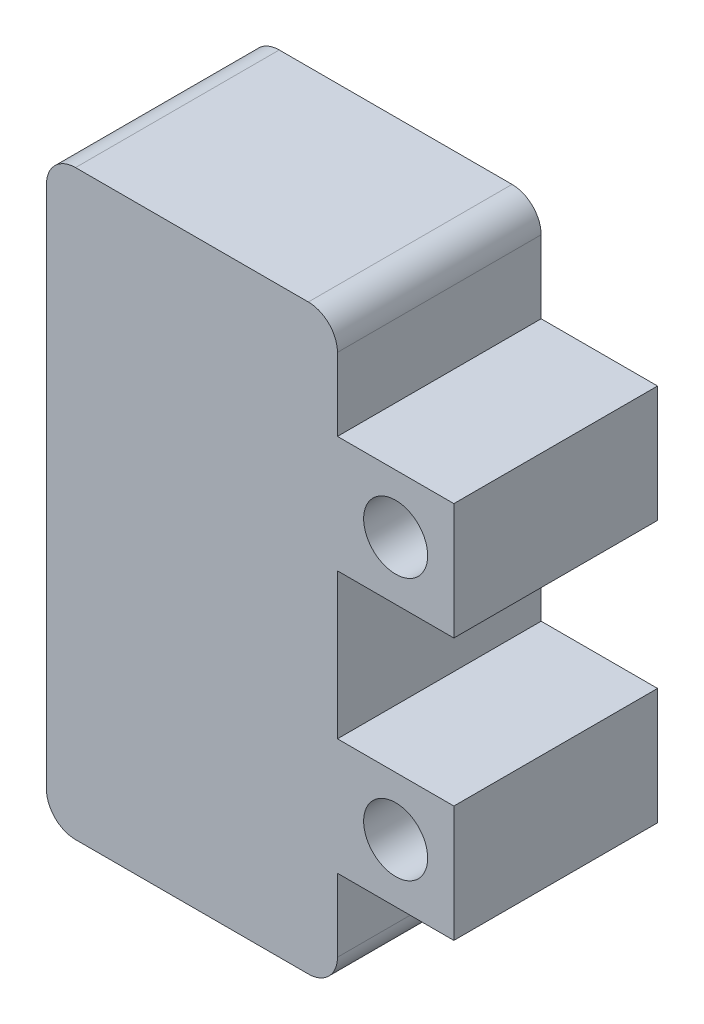
SolidWorks part; units mm, degrees
ref_plane "前视基准面" through (0, 0, 0) normal (0, 0, 1) x (1, 0, 0)
ref_plane "上视基准面" through (0, 0, 0) normal (0, 1, 0) x (1, 0, 0)
ref_plane "右视基准面" through (0, 0, 0) normal (1, 0, 0) x (0, 0, -1)
sketch "草图1" plane through (0, 0, 0) normal (0, 0, 1) x (1, 0, 0)
  line L1 (-5, 10) -> (5, 10)
  line L2 (-5, 10) -> (-5, -10)
  line L3 (-5, -10) -> (5, -10)
  line L4 (5, 10) -> (5, -10)
  line L5 (-5, 10) -> (5, -10) construction
  line L6 (-5, -10) -> (5, 10) construction
  point P0 (0, 0)
  dimension "D1" = 10
  dimension "D2" = 20
extrude "凸台-拉伸1" add sketch "草图1" along normal blind 7
sketch "草图2" plane through (0, 0, 7) normal (0, 0, 1) x (1, 0, 0)
  line L0 (5, -10) -> (5, 10) construction
  line L1 (5, 6.5) -> (9, 6.5)
  line L2 (5, 6.5) -> (5, 2.5)
  line L3 (5, 2.5) -> (9, 2.5)
  line L4 (9, 6.5) -> (9, 2.5)
  line L5 (-5, 0) -> (5, 0) construction
  line L6 (5, -2.5) -> (9, -2.5)
  line L7 (5, -2.5) -> (5, -6.5)
  line L8 (5, -6.5) -> (9, -6.5)
  line L9 (9, -2.5) -> (9, -6.5)
  line L10 (-5, 10) -> (-5, -10) construction
  line L11 (5, 4.5) -> (9, 4.5) construction
  line L12 (7, 6.5) -> (7, 2.5) construction
  line L13 (5, -4.5) -> (9, -4.5) construction
  line L14 (7, -2.5) -> (7, -6.5) construction
  circle A0 centre (7, 4.5) radius 1.1
  circle A1 centre (7, -4.5) radius 1.1
  dimension "D5" = 2.2
  dimension "D3" = 9
  dimension "D1" = 4
  dimension "D2" = 4
extrude "凸台-拉伸2" add sketch "草图2" against normal blind 7
fillet "圆角1" radius 1 4 edges at (5, -10, 3.5) (-5, -10, 3.5) (5, 10, 3.5) (-5, 10, 3.5)
sketch "草图3" plane through (-5, 0, 0) normal (-1, 0, 0) x (0, 0, 1)
  line L1 (0.5738, 8.4382) -> (6.5282, 8.4382)
  line L2 (0.5738, 8.4382) -> (0.5738, 5.7843)
  line L3 (0.5738, 5.7843) -> (6.5282, 5.7843)
  line L4 (6.5282, 8.4382) -> (6.5282, 5.7843)
extrude "切除-拉伸1" cut sketch "草图3" against normal blind 0.1
mirror "镜向1" about plane through (0, 0, 0) normal (0, 1, 0) of "切除-拉伸1"
